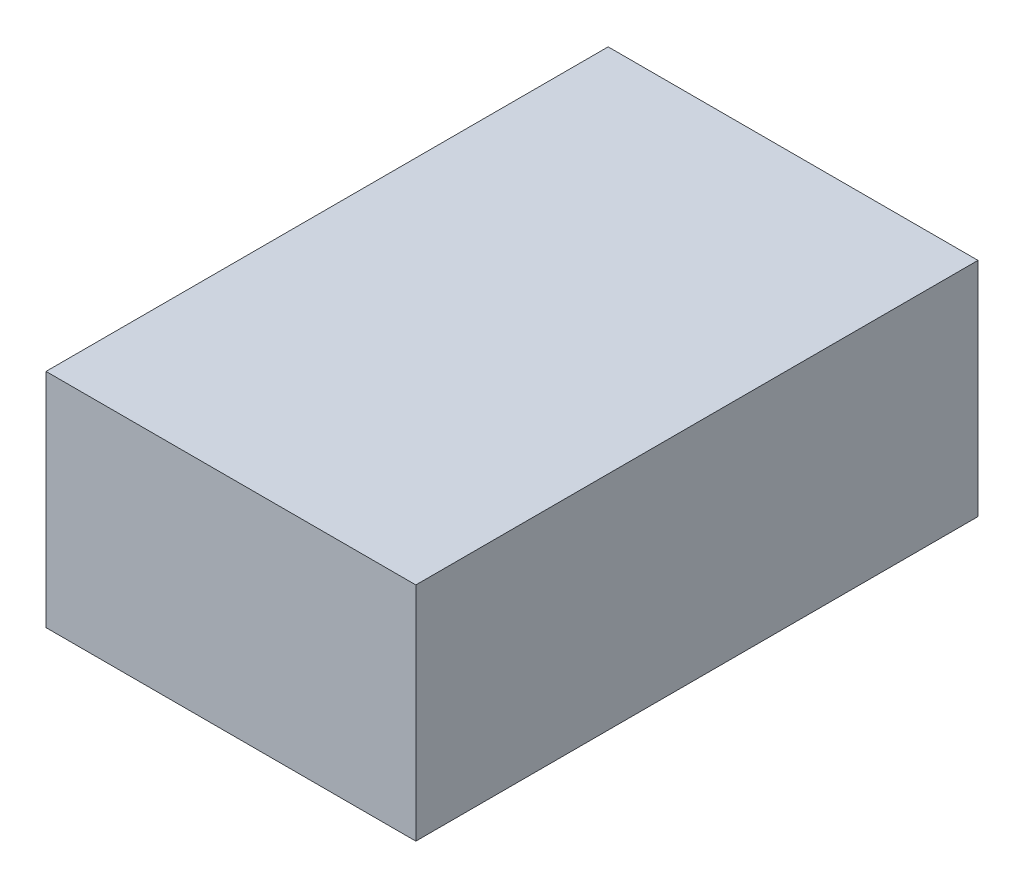
from build123d import *

# Parameters (mm, degrees)
SKETCH1_W           = 50
SKETCH1_H           = 30
BOSS_EXTRUDE1_DEPTH = 76


with BuildPart() as part:
    # Sketch1 → Boss-Extrude1 (new body)
    with BuildSketch(Plane.XY):
        Rectangle(SKETCH1_W, SKETCH1_H)
    extrude(amount=BOSS_EXTRUDE1_DEPTH)


solid = part.part
